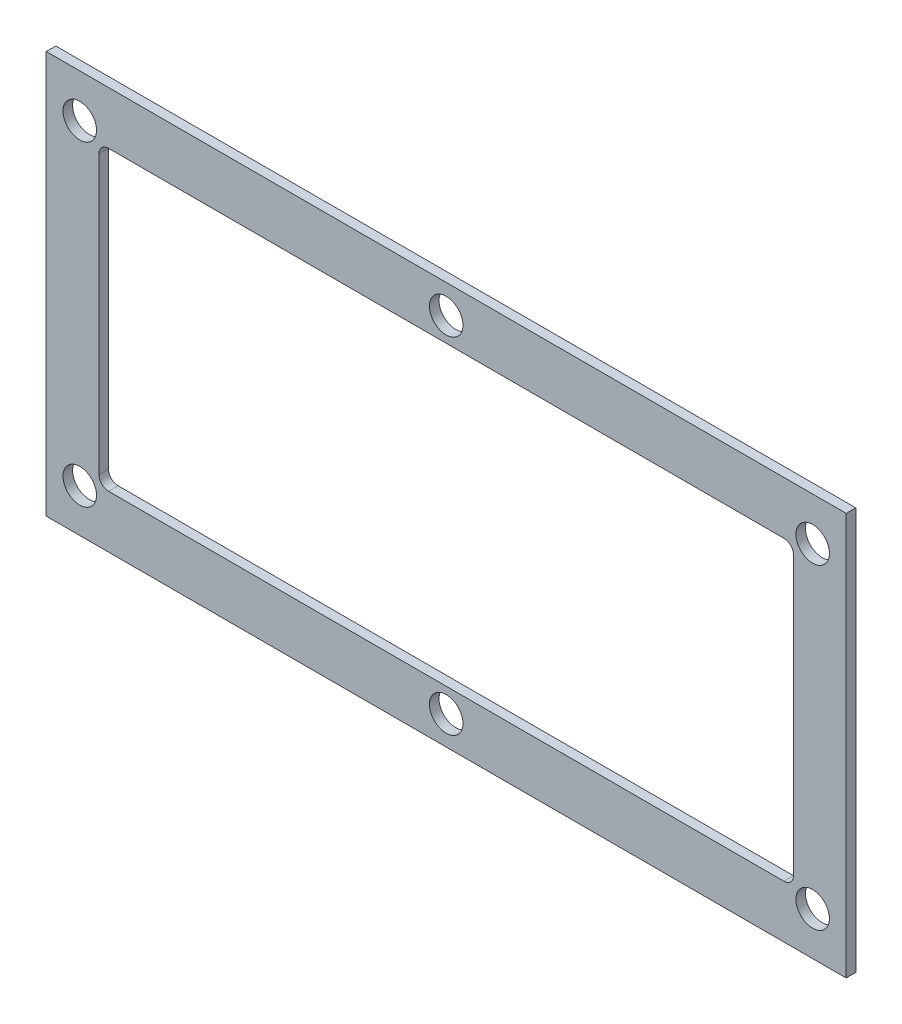
SolidWorks part; units mm, degrees
ref_plane "Front Plane" through (0, 0, 0) normal (0, 0, 1) x (1, 0, 0)
ref_plane "Top Plane" through (0, 0, 0) normal (0, 1, 0) x (1, 0, 0)
ref_plane "Right Plane" through (0, 0, 0) normal (1, 0, 0) x (0, 0, -1)
sketch "Sketch1" plane through (0, 0, 0) normal (0, 0, 1) x (1, 0, 0)
  line L1 (41.75, -21) -> (-41.75, -21)
  line L2 (41.75, -21) -> (41.75, 21)
  line L3 (41.75, 21) -> (-41.75, 21)
  line L4 (-41.75, -21) -> (-41.75, 21)
  line L5 (41.75, -21) -> (-41.75, 21) construction
  line L6 (41.75, 21) -> (-41.75, -21) construction
  line L7 (36.25, -15.5) -> (-36.25, -15.5)
  line L8 (36.25, -15.5) -> (36.25, 15.5)
  line L9 (36.25, 15.5) -> (-36.25, 15.5)
  line L10 (-36.25, -15.5) -> (-36.25, 15.5)
  line L11 (36.25, -15.5) -> (-36.25, 15.5) construction
  line L12 (36.25, 15.5) -> (-36.25, -15.5) construction
  circle A0 centre (-38.25, 16.5) radius 1.75
  circle A1 centre (38.25, 16.5) radius 1.75
  circle A2 centre (38.25, -16.5) radius 1.75
  circle A3 centre (-38.25, -16.5) radius 1.75
  circle A4 centre (0, 18) radius 1.75
  circle A5 centre (0, -18) radius 1.75
  point P0 (0, 0)
  point P18 (0, 0)
  dimension "D3" = 3.5
  dimension "D6" = 3.5
  dimension "D7" = 3.5
  dimension "D8" = 3.5
  dimension "D11" = 3.5
  dimension "D12" = 3.5
  dimension "D1" = 42
  dimension "D2" = 83.5
  dimension "D4" = 3.5
  dimension "D5" = 4.5
  dimension "D9" = 3.5
  dimension "D10" = 4.5
  dimension "D13" = 3
  dimension "D14" = 3
  dimension "D15" = 31
  dimension "D16" = 72.5
extrude "Boss-Extrude1" add sketch "Sketch1" along normal blind 1
fillet "Fillet1" radius 1 4 edges at (36.25, 15.5, 0.5) (36.25, -15.5, 0.5) (-36.25, -15.5, 0.5) (-36.25, 15.5, 0.5)
